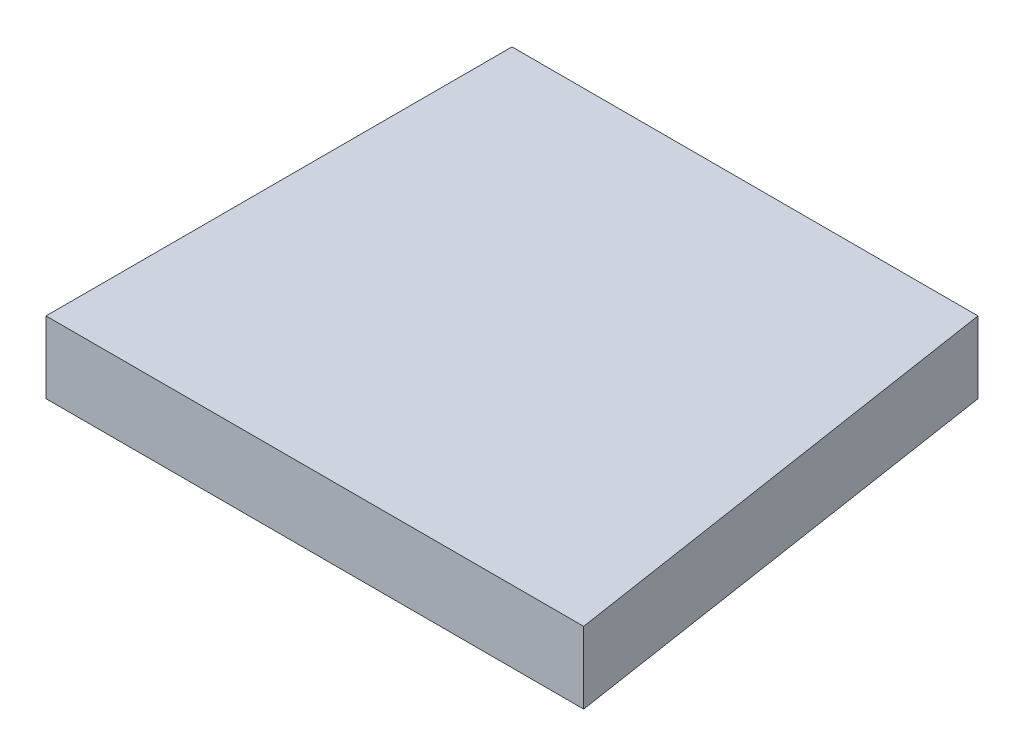
SolidWorks part; units mm, degrees
material "A3"
ref_plane "前视基准面" through (0, 0, 0) normal (0, 0, 1) x (1, 0, 0)
ref_plane "上视基准面" through (0, 0, 0) normal (0, 1, 0) x (1, 0, 0)
ref_plane "右视基准面" through (0, 0, 0) normal (1, 0, 0) x (0, 0, -1)
sketch "草图1" plane through (0, 0, 0) normal (0, 1, 0) x (1, 0, 0)
  line L0 (0, 0) -> (0, 26)
  line L1 (0, 26) -> (26, 26)
  line L2 (26, 26) -> (30, 0)
  line L3 (30, 0) -> (0, 0)
  dimension "D1" = 26
  dimension "D2" = 26
  dimension "D3" = 30
extrude "凸台-拉伸1" add sketch "草图1" along normal blind 4
